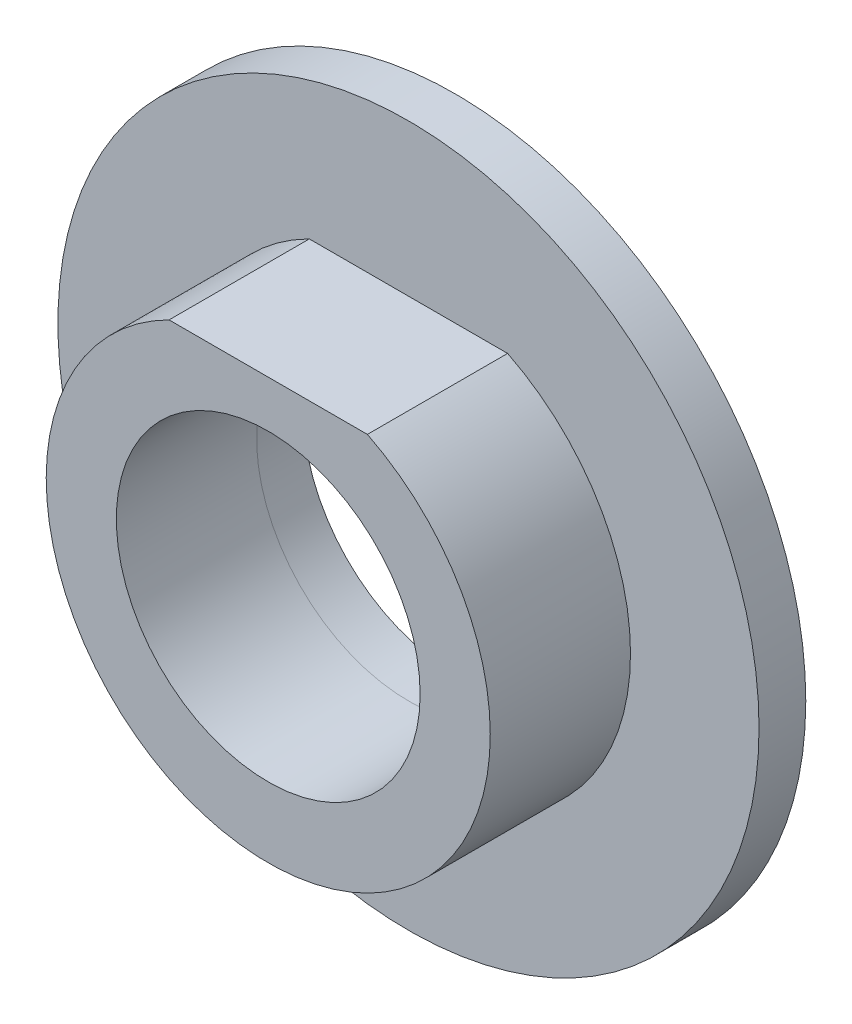
SolidWorks part; units mm, degrees
ref_plane "前视基准面" through (0, 0, 0) normal (0, 0, 1) x (1, 0, 0)
ref_plane "上视基准面" through (0, 0, 0) normal (0, 1, 0) x (1, 0, 0)
ref_plane "右视基准面" through (0, 0, 0) normal (1, 0, 0) x (0, 0, -1)
sketch "草图1" plane through (0, 0, 0) normal (0, 0, 1) x (1, 0, 0)
  circle A0 centre (0, 0) radius 15
  dimension "D1" = 30
extrude "凸台-拉伸1" add sketch "草图1" along normal blind 2
sketch "草图2" plane through (0, 0, 2) normal (0, 0, 1) x (1, 0, 0)
  circle A0 centre (0, 0) radius 9.5
  dimension "D1" = 19
extrude "凸台-拉伸2" add sketch "草图2" along normal blind 6 separate body
sketch "草图3" plane through (0, 0, 8) normal (0, 0, 1) x (1, 0, 0)
  circle A1 centre (0, 0) radius 6.5
  dimension "D1" = 13
extrude "切除-拉伸1" cut sketch "草图3" against normal blind 15
sketch "草图4" plane through (0, 0, 8) normal (0, 0, 1) x (1, 0, 0)
  line L1 (0, -9.5) -> (0, 8.5) construction
  line L2 (-4.2426, 8.5) -> (4.2426, 8.5)
  arc A0 (4.2426, 8.5) -> (-4.2426, 8.5) centre (0, 0) ccw
  circle A1 centre (0, 0) radius 9.5 construction
  point P10 (0, 8.5)
  dimension "D2" = 19
  dimension "D3" = 18
extrude "切除-拉伸2" cut sketch "草图4" against normal up to surface (6 mm away) up to face at (6.5, 0, 2)
